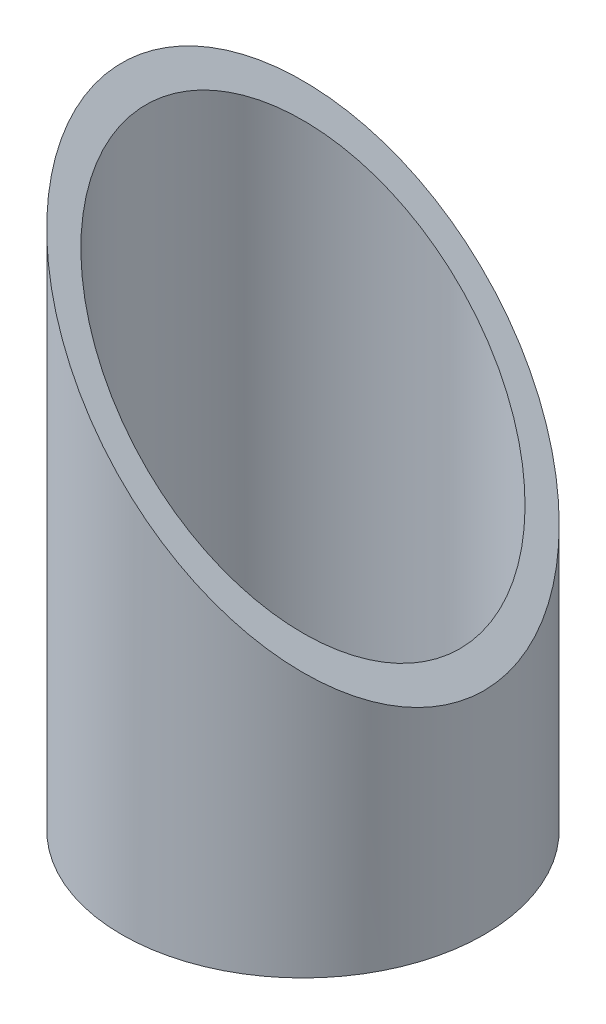
SolidWorks part; units mm, degrees
material "Q235"
ref_plane "Front Plane" through (0, 0, 0) normal (0, 0, 1) x (1, 0, 0)
ref_plane "Top Plane" through (0, 0, 0) normal (0, 1, 0) x (1, 0, 0)
ref_plane "Right Plane" through (0, 0, 0) normal (1, 0, 0) x (0, 0, -1)
sketch "Sketch1" plane through (0, 0, 0) normal (0, 1, 0) x (1, 0, 0)
  circle A0 centre (0, 0) radius 30
  circle A1 centre (0, 0) radius 26
  dimension "D1" = 4
  dimension "D2" = 60
extrude "Boss-Extrude1" add sketch "Sketch1" along normal blind 95
sketch "Sketch2" plane through (0, 0, 0) normal (0, 0, 1) x (1, 0, 0)
  line L0 (-30, 95) -> (45.7123, 19.2877)
  line L1 (30, 95) -> (-30, 95) construction
  dimension "D1" = 45
extrude "Cut-Extrude1" cut sketch "Sketch2" against normal through all both and the other way through all
